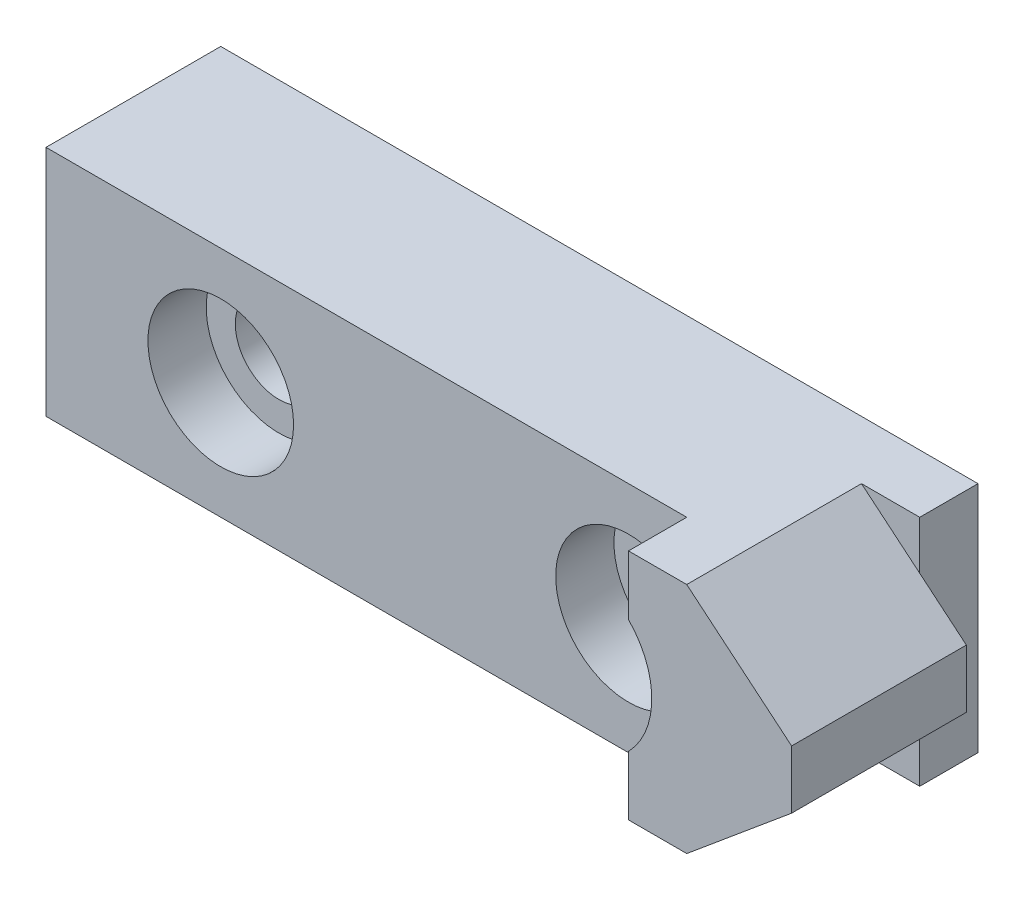
SolidWorks part; units mm, degrees
ref_plane "Front Plane" through (0, 0, 0) normal (0, 0, 1) x (1, 0, 0)
ref_plane "Top Plane" through (0, 0, 0) normal (0, 1, 0) x (1, 0, 0)
ref_plane "Right Plane" through (0, 0, 0) normal (1, 0, 0) x (0, 0, -1)
sketch "Sketch1" plane through (0, 0, 0) normal (0, 0, 1) x (1, 0, 0)
  line L1 (-65, 20) -> (65, 20)
  line L2 (-65, 20) -> (-65, -20)
  line L3 (-65, -20) -> (65, -20)
  line L4 (65, 20) -> (65, -20)
  line L5 (-65, 20) -> (65, -20) construction
  line L6 (-65, -20) -> (65, 20) construction
  point P0 (0, 0)
  dimension "D1" = 40
  dimension "D2" = 130
extrude "Boss-Extrude1" add sketch "Sketch1" along normal blind 10
sketch "Sketch2" plane through (0, 0, 10) normal (0, 0, 1) x (1, 0, 0)
  line L0 (-65, 20) -> (55, 20)
  line L1 (55, 20) -> (73, 5)
  line L2 (73, 5) -> (73, -5)
  line L3 (-65, 20) -> (-65, -20)
  line L4 (-65, -20) -> (55, -20)
  line L5 (55, -20) -> (73, -5)
  line L6 (65, -20) -> (65, 20) construction
  dimension "D1" = 10
  dimension "D2" = 10
  dimension "D3" = 15
  dimension "D4" = 15
  dimension "D5" = 18
extrude "Boss-Extrude2" add sketch "Sketch2" along normal blind 30
sketch "Sketch3" plane through (0, -20, 0) normal (0, -1, 0) x (1, 0, 0)
  line L0 (-65, 40) -> (-65, 0) construction
  line L1 (-65, 30) -> (45, 30)
  line L2 (-65, 30) -> (-65, 40)
  line L3 (-65, 40) -> (45, 40)
  line L4 (45, 30) -> (45, 40)
  line L5 (-65, 40) -> (55, 40) construction
  dimension "D1" = 110
  dimension "D2" = 10
extrude "Cut-Extrude1" cut sketch "Sketch3" against normal blind 40
sketch "Sketch4" plane through (0, 0, 0) normal (0, 0, -1) x (-1, 0, 0)
  line L0 (-65, -11.6667) -> (-65, 11.6667) construction
  line L1 (65, 20) -> (65, -20) construction
  circle A0 centre (-35, 0) radius 7.5
  circle A1 centre (35, 0) radius 7.5
  dimension "D1" = 15
  dimension "D2" = 15
  dimension "D3" = 30
  dimension "D4" = 30
extrude "Cut-Extrude2" cut sketch "Sketch4" against normal blind 40
sketch "Sketch5" plane through (0, 0, 30) normal (0, 0, 1) x (1, 0, 0)
  circle A0 centre (-35, 0) radius 14
  circle A1 centre (35, 0) radius 14
  dimension "D1" = 28
  dimension "D2" = 28
extrude "Cut-Extrude3" cut sketch "Sketch5" along normal blind 40
sketch "Sketch6" plane through (0, 0, 30) normal (0, 0, 1) x (1, 0, 0)
  circle A0 centre (35, 0) radius 12.5
  circle A1 centre (-35, 0) radius 12.5
  dimension "D1" = 25
  dimension "D2" = 25
extrude "Cut-Extrude4" cut sketch "Sketch6" against normal blind 10
